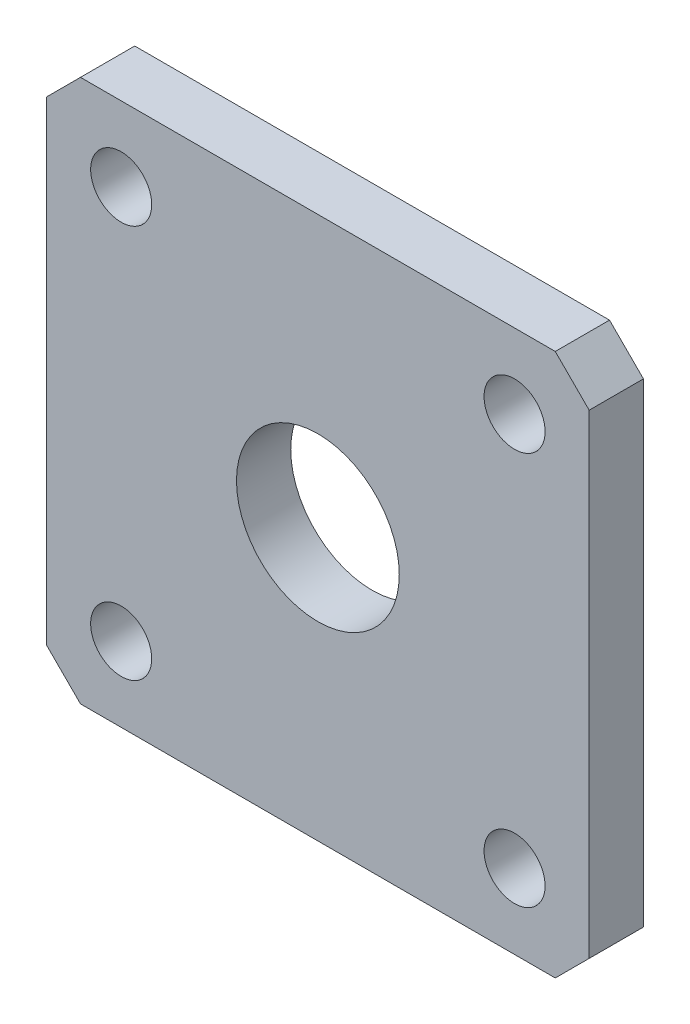
SolidWorks part; units mm, degrees
ref_plane "Front Plane" through (0, 0, 0) normal (0, 0, 1) x (1, 0, 0)
ref_plane "Top Plane" through (0, 0, 0) normal (0, 1, 0) x (1, 0, 0)
ref_plane "Right Plane" through (0, 0, 0) normal (1, 0, 0) x (0, 0, -1)
sketch "Sketch1" plane through (0, 0, 0) normal (0, 0, 1) x (1, 0, 0)
  line L0 (-1.1144, 67.8195) -> (-1.1144, -47.6692) construction
  line L1 (-41.1144, 49.4737) -> (38.8856, 49.4737)
  line L2 (-41.1144, 49.4737) -> (-41.1144, -30.5263)
  line L3 (-41.1144, -30.5263) -> (38.8856, -30.5263)
  line L4 (38.8856, 49.4737) -> (38.8856, -30.5263)
  line L5 (-66.6783, 9.4737) -> (65.051, 9.4737) construction
  line L7 (-30.1144, -19.5263) -> (27.8856, -19.5263) construction
  line L8 (-30.1144, -19.5263) -> (-30.1144, 38.4737) construction
  line L9 (-30.1144, 38.4737) -> (27.8856, 38.4737) construction
  line L10 (27.8856, -19.5263) -> (27.8856, 38.4737) construction
  line L11 (-30.1144, -19.5263) -> (27.8856, 38.4737) construction
  line L12 (-30.1144, 38.4737) -> (27.8856, -19.5263) construction
  circle A0 centre (-1.1144, 9.4737) radius 12
  circle A1 centre (-30.1144, 38.4737) radius 4.5
  circle A2 centre (-30.1144, -19.5263) radius 4.5
  circle A3 centre (27.8856, -19.5263) radius 4.5
  circle A4 centre (27.8856, 38.4737) radius 4.5
  point P8 (-1.1144, 9.4737)
  dimension "D1" = 80
  dimension "D2" = 80
  dimension "D3" = 58
  dimension "D4" = 58
  dimension "D5" = 11
  dimension "D6" = 11
extrude "Boss-Extrude1" add sketch "Sketch1" along normal blind 8
chamfer "Chamfer1" distance 5 angle 45 4 edges at (38.8856, -30.5263, 4) (38.8856, 49.4737, 4) (-41.1144, -30.5263, 4) (-41.1144, 49.4737, 4)
